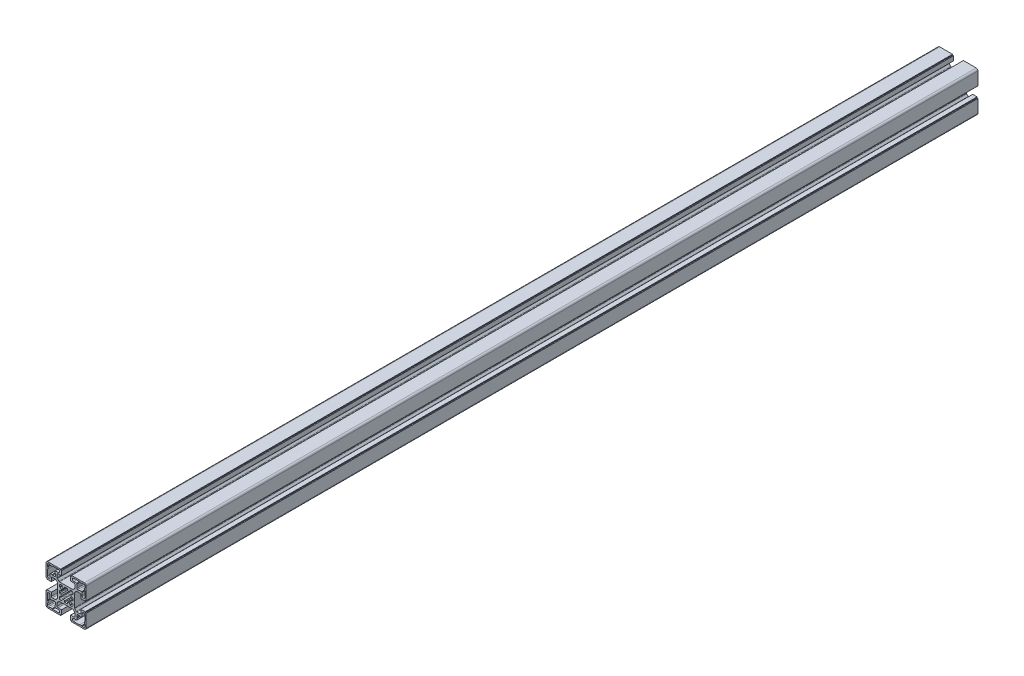
from build123d import *

# Parameters (mm, degrees)
EXTRUDE_1_DEPTH = 1000


with BuildPart() as part:
    # 草图1 → 拉伸1 (new body)
    with BuildSketch(Plane.XY):
        with BuildLine():
            Line((33.706586033, 40.501982097), (35.388566549, 38.820001582))
            ThreePointArc((35.388566549, 38.820001582), (35.712989897, 38.603228831), (36.09567333, 38.527108363))
            Line((36.09567333, 38.527108363), (39.413692815, 38.527108363))
            ThreePointArc((39.413692815, 38.527108363), (40.120799596, 38.820001582), (40.413692815, 39.527108363))
            Line((40.413692815, 39.527108363), (40.413692815, 43.427108363))
            Line((40.413692815, 43.427108363), (45.413692815, 43.427108363))
            Line((45.413692815, 43.427108363), (45.413692815, 42.427108363))
            Line((45.413692815, 42.427108363), (46.413692815, 42.427108363))
            Line((46.413692815, 42.427108363), (46.413692815, 28.027108363))
            ThreePointArc((46.413692815, 28.027108363), (45.827906377, 26.612894801), (44.413692815, 26.027108363))
            Line((44.413692815, 26.027108363), (30.013692814, 26.027108363))
            Line((30.013692814, 26.027108363), (30.013692814, 27.027108363))
            Line((30.013692814, 27.027108363), (29.013692814, 27.027108363))
            Line((29.013692814, 27.027108363), (29.013692814, 32.027108363))
            Line((29.013692814, 32.027108363), (32.913692814, 32.027108363))
            ThreePointArc((32.913692814, 32.027108363), (33.620799596, 32.320001582), (33.913692814, 33.027108363))
            Line((33.913692814, 33.027108363), (33.913692814, 36.345127848))
            ThreePointArc((33.913692814, 36.345127848), (33.837572347, 36.72781128), (33.620799596, 37.052234629))
            Line((33.620799596, 37.052234629), (31.938819081, 38.734215144))
            ThreePointArc((31.938819081, 38.734215144), (31.614395732, 38.950987895), (31.231712299, 39.027108363))
            Line((31.231712299, 39.027108363), (16.59567333, 39.027108363))
            ThreePointArc((16.59567333, 39.027108363), (16.212989897, 38.950987895), (15.888566548, 38.734215144))
            Line((15.888566548, 38.734215144), (14.206586033, 37.052234629))
            ThreePointArc((14.206586033, 37.052234629), (13.989813282, 36.72781128), (13.913692814, 36.345127848))
            Line((13.913692814, 36.345127848), (13.913692814, 33.027108363))
            ThreePointArc((13.913692814, 33.027108363), (14.206586033, 32.320001582), (14.913692814, 32.027108363))
            Line((14.913692814, 32.027108363), (18.813692815, 32.027108363))
            Line((18.813692815, 32.027108363), (18.813692815, 27.027108363))
            Line((18.813692815, 27.027108363), (17.813692815, 27.027108363))
            Line((17.813692815, 27.027108363), (17.813692815, 26.027108363))
            Line((17.813692815, 26.027108363), (3.413692814, 26.027108363))
            ThreePointArc((3.413692814, 26.027108363), (1.999479252, 26.612894801), (1.413692814, 28.027108363))
            Line((1.413692814, 28.027108363), (1.413692814, 42.427108363))
            Line((1.413692814, 42.427108363), (2.413692814, 42.427108363))
            Line((2.413692814, 42.427108363), (2.413692814, 43.427108363))
            Line((2.413692814, 43.427108363), (7.413692814, 43.427108363))
            Line((7.413692814, 43.427108363), (7.413692814, 39.527108363))
            ThreePointArc((7.413692814, 39.527108363), (7.706586033, 38.820001582), (8.413692814, 38.527108363))
            Line((8.413692814, 38.527108363), (11.731712299, 38.527108363))
            ThreePointArc((11.731712299, 38.527108363), (12.114395732, 38.603228831), (12.43881908, 38.820001582))
            Line((12.43881908, 38.820001582), (14.120799595, 40.501982097))
            ThreePointArc((14.120799595, 40.501982097), (14.337572347, 40.826405446), (14.413692814, 41.209088878))
            Line((14.413692814, 41.209088878), (14.413692814, 55.845127848))
            ThreePointArc((14.413692814, 55.845127848), (14.337572347, 56.22781128), (14.120799595, 56.552234629))
            Line((14.120799595, 56.552234629), (12.43881908, 58.234215144))
            ThreePointArc((12.43881908, 58.234215144), (12.114395732, 58.450987896), (11.731712299, 58.527108363))
            Line((11.731712299, 58.527108363), (8.413692814, 58.527108363))
            ThreePointArc((8.413692814, 58.527108363), (7.706586033, 58.234215144), (7.413692814, 57.527108363))
            Line((7.413692814, 57.527108363), (7.413692814, 53.627108363))
            Line((7.413692814, 53.627108363), (2.413692814, 53.627108363))
            Line((2.413692814, 53.627108363), (2.413692814, 54.627108363))
            Line((2.413692814, 54.627108363), (1.413692814, 54.627108363))
            Line((1.413692814, 54.627108363), (1.413692814, 69.027108363))
            ThreePointArc((1.413692814, 69.027108363), (1.999479252, 70.441321926), (3.413692814, 71.027108363))
            Line((3.413692814, 71.027108363), (17.813692815, 71.027108363))
            Line((17.813692815, 71.027108363), (17.813692815, 70.027108363))
            Line((17.813692815, 70.027108363), (18.813692815, 70.027108363))
            Line((18.813692815, 70.027108363), (18.813692815, 65.027108363))
            Line((18.813692815, 65.027108363), (14.913692814, 65.027108363))
            ThreePointArc((14.913692814, 65.027108363), (14.206586033, 64.734215145), (13.913692814, 64.027108363))
            Line((13.913692814, 64.027108363), (13.913692814, 60.709088878))
            ThreePointArc((13.913692814, 60.709088878), (13.989813282, 60.326405446), (14.206586033, 60.001982097))
            Line((14.206586033, 60.001982097), (15.888566548, 58.320001582))
            ThreePointArc((15.888566548, 58.320001582), (16.212989897, 58.103228831), (16.59567333, 58.027108363))
            Line((16.59567333, 58.027108363), (31.231712299, 58.027108363))
            ThreePointArc((31.231712299, 58.027108363), (31.614395732, 58.103228831), (31.938819081, 58.320001582))
            Line((31.938819081, 58.320001582), (33.620799596, 60.001982097))
            ThreePointArc((33.620799596, 60.001982097), (33.837572347, 60.326405446), (33.913692814, 60.709088878))
            Line((33.913692814, 60.709088878), (33.913692814, 64.027108363))
            ThreePointArc((33.913692814, 64.027108363), (33.620799596, 64.734215145), (32.913692814, 65.027108363))
            Line((32.913692814, 65.027108363), (29.013692814, 65.027108363))
            Line((29.013692814, 65.027108363), (29.013692814, 70.027108363))
            Line((29.013692814, 70.027108363), (30.013692814, 70.027108363))
            Line((30.013692814, 70.027108363), (30.013692814, 71.027108363))
            Line((30.013692814, 71.027108363), (44.413692815, 71.027108363))
            ThreePointArc((44.413692815, 71.027108363), (45.827906377, 70.441321926), (46.413692815, 69.027108363))
            Line((46.413692815, 69.027108363), (46.413692815, 54.627108363))
            Line((46.413692815, 54.627108363), (45.413692815, 54.627108363))
            Line((45.413692815, 54.627108363), (45.413692815, 53.627108363))
            Line((45.413692815, 53.627108363), (40.413692815, 53.627108363))
            Line((40.413692815, 53.627108363), (40.413692815, 57.527108363))
            ThreePointArc((40.413692815, 57.527108363), (40.120799596, 58.234215144), (39.413692815, 58.527108363))
            Line((39.413692815, 58.527108363), (36.09567333, 58.527108363))
            ThreePointArc((36.09567333, 58.527108363), (35.712989897, 58.450987896), (35.388566549, 58.234215144))
            Line((35.388566549, 58.234215144), (33.706586033, 56.552234629))
            ThreePointArc((33.706586033, 56.552234629), (33.489813282, 56.22781128), (33.413692815, 55.845127848))
            Line((33.413692815, 55.845127848), (33.413692815, 41.209088878))
            ThreePointArc((33.413692815, 41.209088878), (33.489813282, 40.826405446), (33.706586033, 40.501982097))
        make_face()
        with BuildLine():
            Line((30.535013158, 44.027108363), (29.082272168, 45.479849354))
            ThreePointArc((29.082272168, 45.479849354), (29.45697001, 46.231007769), (29.723167834, 47.027108363))
            Line((29.723167834, 47.027108363), (31.413692814, 47.027108363))
            Line((31.413692814, 47.027108363), (31.413692814, 50.027108363))
            Line((31.413692814, 50.027108363), (29.723167834, 50.027108363))
            ThreePointArc((29.723167834, 50.027108363), (29.45697001, 50.823208957), (29.082272168, 51.574367373))
            Line((29.082272168, 51.574367373), (30.535013158, 53.027108363))
            Line((30.535013158, 53.027108363), (31.413692814, 53.027108363))
            Line((31.413692814, 53.027108363), (31.413692814, 55.027108363))
            ThreePointArc((31.413692814, 55.027108363), (31.120799596, 55.734215144), (30.413692814, 56.027108363))
            Line((30.413692814, 56.027108363), (28.413692814, 56.027108363))
            Line((28.413692814, 56.027108363), (28.413692814, 55.148428707))
            Line((28.413692814, 55.148428707), (26.960951824, 53.695687716))
            ThreePointArc((26.960951824, 53.695687716), (26.209793409, 54.070385558), (25.413692814, 54.336583382))
            Line((25.413692814, 54.336583382), (25.413692814, 56.027108363))
            Line((25.413692814, 56.027108363), (22.413692814, 56.027108363))
            Line((22.413692814, 56.027108363), (22.413692814, 54.336583382))
            ThreePointArc((22.413692814, 54.336583382), (21.61759222, 54.070385558), (20.866433805, 53.695687716))
            Line((20.866433805, 53.695687716), (19.413692814, 55.148428707))
            Line((19.413692814, 55.148428707), (19.413692814, 56.027108363))
            Line((19.413692814, 56.027108363), (17.413692814, 56.027108363))
            ThreePointArc((17.413692814, 56.027108363), (16.706586033, 55.734215144), (16.413692814, 55.027108363))
            Line((16.413692814, 55.027108363), (16.413692814, 53.027108363))
            Line((16.413692814, 53.027108363), (17.292372471, 53.027108363))
            Line((17.292372471, 53.027108363), (18.745113461, 51.574367373))
            ThreePointArc((18.745113461, 51.574367373), (18.370415619, 50.823208957), (18.104217795, 50.027108363))
            Line((18.104217795, 50.027108363), (16.413692814, 50.027108363))
            Line((16.413692814, 50.027108363), (16.413692814, 47.027108363))
            Line((16.413692814, 47.027108363), (18.104217795, 47.027108363))
            ThreePointArc((18.104217795, 47.027108363), (18.370415619, 46.231007769), (18.745113461, 45.479849354))
            Line((18.745113461, 45.479849354), (17.292372471, 44.027108363))
            Line((17.292372471, 44.027108363), (16.413692814, 44.027108363))
            Line((16.413692814, 44.027108363), (16.413692814, 42.027108363))
            ThreePointArc((16.413692814, 42.027108363), (16.706586033, 41.320001582), (17.413692814, 41.027108363))
            Line((17.413692814, 41.027108363), (19.413692814, 41.027108363))
            Line((19.413692814, 41.027108363), (19.413692814, 41.90578802))
            Line((19.413692814, 41.90578802), (20.866433805, 43.35852901))
            ThreePointArc((20.866433805, 43.35852901), (21.61759222, 42.983831168), (22.413692814, 42.717633344))
            Line((22.413692814, 42.717633344), (22.413692814, 41.027108363))
            Line((22.413692814, 41.027108363), (25.413692814, 41.027108363))
            Line((25.413692814, 41.027108363), (25.413692814, 42.717633344))
            ThreePointArc((25.413692814, 42.717633344), (26.209793409, 42.983831168), (26.960951824, 43.35852901))
            Line((26.960951824, 43.35852901), (28.413692814, 41.90578802))
            Line((28.413692814, 41.90578802), (28.413692814, 41.027108363))
            Line((28.413692814, 41.027108363), (30.413692814, 41.027108363))
            ThreePointArc((30.413692814, 41.027108363), (31.120799596, 41.320001582), (31.413692814, 42.027108363))
            Line((31.413692814, 42.027108363), (31.413692814, 44.027108363))
            Line((31.413692814, 44.027108363), (30.535013158, 44.027108363))
        make_face(mode=Mode.SUBTRACT)
        with BuildLine():
            Line((11.413692814, 66.027108363), (11.913692814, 66.527108364))
            Line((11.913692814, 66.527108364), (15.313692814, 66.527108364))
            ThreePointArc((15.313692814, 66.527108364), (16.813692814, 68.027108363), (15.313692814, 69.527108363))
            Line((15.313692814, 69.527108363), (8.913692815, 69.527108363))
            Line((8.913692815, 69.527108363), (8.413692814, 69.027108363))
            Line((8.413692814, 69.027108363), (6.413692814, 69.027108363))
            Line((6.413692814, 69.027108363), (5.913692814, 69.527108363))
            Line((5.913692814, 69.527108363), (3.913692814, 69.527108363))
            ThreePointArc((3.913692814, 69.527108363), (3.206586033, 69.234215145), (2.913692814, 68.527108363))
            Line((2.913692814, 68.527108363), (2.913692814, 66.527108363))
            Line((2.913692814, 66.527108363), (3.413692814, 66.027108363))
            Line((3.413692814, 66.027108363), (3.413692814, 64.027108363))
            Line((3.413692814, 64.027108363), (2.913692814, 63.527108363))
            Line((2.913692814, 63.527108363), (2.913692814, 57.127108364))
            ThreePointArc((2.913692814, 57.127108364), (4.413692814, 55.627108364), (5.913692814, 57.127108364))
            Line((5.913692814, 57.127108364), (5.913692814, 60.527108363))
            Line((5.913692814, 60.527108363), (6.413692814, 61.027108363))
            Line((6.413692814, 61.027108363), (8.413692814, 61.027108363))
            Line((8.413692814, 61.027108363), (8.913692814, 60.527108363))
            Line((8.913692814, 60.527108363), (10.913692814, 60.527108363))
            ThreePointArc((10.913692814, 60.527108363), (11.620799595, 60.820001582), (11.913692814, 61.527108363))
            Line((11.913692814, 61.527108363), (11.913692814, 63.527108363))
            Line((11.913692814, 63.527108363), (11.413692814, 64.027108363))
            Line((11.413692814, 64.027108363), (11.413692814, 66.027108363))
        make_face(mode=Mode.SUBTRACT)
        with BuildLine():
            Line((11.913692815, 30.527108363), (11.413692814, 31.027108363))
            Line((11.413692814, 31.027108363), (11.413692814, 33.027108363))
            Line((11.413692814, 33.027108363), (11.913692815, 33.527108363))
            Line((11.913692815, 33.527108363), (11.913692815, 35.527108363))
            ThreePointArc((11.913692815, 35.527108363), (11.620799596, 36.234215144), (10.913692815, 36.527108363))
            Line((10.913692815, 36.527108363), (8.913692815, 36.527108363))
            Line((8.913692815, 36.527108363), (8.413692815, 36.027108363))
            Line((8.413692815, 36.027108363), (6.413692814, 36.027108363))
            Line((6.413692814, 36.027108363), (5.913692814, 36.527108363))
            Line((5.913692814, 36.527108363), (5.913692814, 39.927108363))
            ThreePointArc((5.913692814, 39.927108363), (4.413692814, 41.427108363), (2.913692814, 39.927108363))
            Line((2.913692814, 39.927108363), (2.913692814, 33.527108363))
            Line((2.913692814, 33.527108363), (3.413692814, 33.027108363))
            Line((3.413692814, 33.027108363), (3.413692814, 31.027108363))
            Line((3.413692814, 31.027108363), (2.913692814, 30.527108363))
            Line((2.913692814, 30.527108363), (2.913692814, 28.527108363))
            ThreePointArc((2.913692814, 28.527108363), (3.206586033, 27.820001582), (3.913692814, 27.527108363))
            Line((3.913692814, 27.527108363), (5.913692814, 27.527108363))
            Line((5.913692814, 27.527108363), (6.413692814, 28.027108363))
            Line((6.413692814, 28.027108363), (8.413692814, 28.027108363))
            Line((8.413692814, 28.027108363), (8.913692815, 27.527108363))
            Line((8.913692815, 27.527108363), (15.313692814, 27.527108363))
            ThreePointArc((15.313692814, 27.527108363), (16.813692814, 29.027108363), (15.313692814, 30.527108363))
            Line((15.313692814, 30.527108363), (11.913692815, 30.527108363))
        make_face(mode=Mode.SUBTRACT)
        with BuildLine():
            Line((41.913692815, 36.527108363), (41.413692815, 36.027108363))
            Line((41.413692815, 36.027108363), (39.413692815, 36.027108363))
            Line((39.413692815, 36.027108363), (38.913692814, 36.527108363))
            Line((38.913692814, 36.527108363), (36.913692815, 36.527108363))
            ThreePointArc((36.913692815, 36.527108363), (36.206586033, 36.234215145), (35.913692815, 35.527108363))
            Line((35.913692815, 35.527108363), (35.913692815, 33.527108364))
            Line((35.913692815, 33.527108364), (36.413692815, 33.027108363))
            Line((36.413692815, 33.027108363), (36.413692815, 31.027108363))
            Line((36.413692815, 31.027108363), (35.913692815, 30.527108363))
            Line((35.913692815, 30.527108363), (32.513692815, 30.527108363))
            ThreePointArc((32.513692815, 30.527108363), (31.013692815, 29.027108363), (32.513692815, 27.527108363))
            Line((32.513692815, 27.527108363), (38.913692814, 27.527108363))
            Line((38.913692814, 27.527108363), (39.413692814, 28.027108363))
            Line((39.413692814, 28.027108363), (41.413692814, 28.027108363))
            Line((41.413692814, 28.027108363), (41.913692815, 27.527108363))
            Line((41.913692815, 27.527108363), (43.913692815, 27.527108363))
            ThreePointArc((43.913692815, 27.527108363), (44.620799596, 27.820001582), (44.913692815, 28.527108363))
            Line((44.913692815, 28.527108363), (44.913692815, 30.527108363))
            Line((44.913692815, 30.527108363), (44.413692814, 31.027108363))
            Line((44.413692814, 31.027108363), (44.413692814, 33.027108363))
            Line((44.413692814, 33.027108363), (44.913692815, 33.527108364))
            Line((44.913692815, 33.527108364), (44.913692815, 39.927108363))
            ThreePointArc((44.913692815, 39.927108363), (43.413692815, 41.427108363), (41.913692815, 39.927108363))
            Line((41.913692815, 39.927108363), (41.913692815, 36.527108363))
        make_face(mode=Mode.SUBTRACT)
        with BuildLine():
            Line((35.913692815, 66.527108363), (36.413692815, 66.027108363))
            Line((36.413692815, 66.027108363), (36.413692815, 64.027108363))
            Line((36.413692815, 64.027108363), (35.913692815, 63.527108363))
            Line((35.913692815, 63.527108363), (35.913692815, 61.527108363))
            ThreePointArc((35.913692815, 61.527108363), (36.206586033, 60.820001582), (36.913692815, 60.527108363))
            Line((36.913692815, 60.527108363), (38.913692814, 60.527108363))
            Line((38.913692814, 60.527108363), (39.413692815, 61.027108364))
            Line((39.413692815, 61.027108364), (41.413692815, 61.027108364))
            Line((41.413692815, 61.027108364), (41.913692815, 60.527108363))
            Line((41.913692815, 60.527108363), (41.913692815, 57.127108364))
            ThreePointArc((41.913692815, 57.127108364), (43.413692815, 55.627108364), (44.913692815, 57.127108364))
            Line((44.913692815, 57.127108364), (44.913692815, 63.527108363))
            Line((44.913692815, 63.527108363), (44.413692815, 64.027108363))
            Line((44.413692815, 64.027108363), (44.413692815, 66.027108363))
            Line((44.413692815, 66.027108363), (44.913692815, 66.527108363))
            Line((44.913692815, 66.527108363), (44.913692815, 68.527108363))
            ThreePointArc((44.913692815, 68.527108363), (44.620799596, 69.234215145), (43.913692815, 69.527108363))
            Line((43.913692815, 69.527108363), (41.913692815, 69.527108363))
            Line((41.913692815, 69.527108363), (41.413692814, 69.027108363))
            Line((41.413692814, 69.027108363), (39.413692814, 69.027108363))
            Line((39.413692814, 69.027108363), (38.913692814, 69.527108363))
            Line((38.913692814, 69.527108363), (32.513692815, 69.527108363))
            ThreePointArc((32.513692815, 69.527108363), (31.013692815, 68.027108363), (32.513692815, 66.527108363))
            Line((32.513692815, 66.527108363), (35.913692815, 66.527108363))
        make_face(mode=Mode.SUBTRACT)
    extrude(amount=EXTRUDE_1_DEPTH)


solid = part.part
